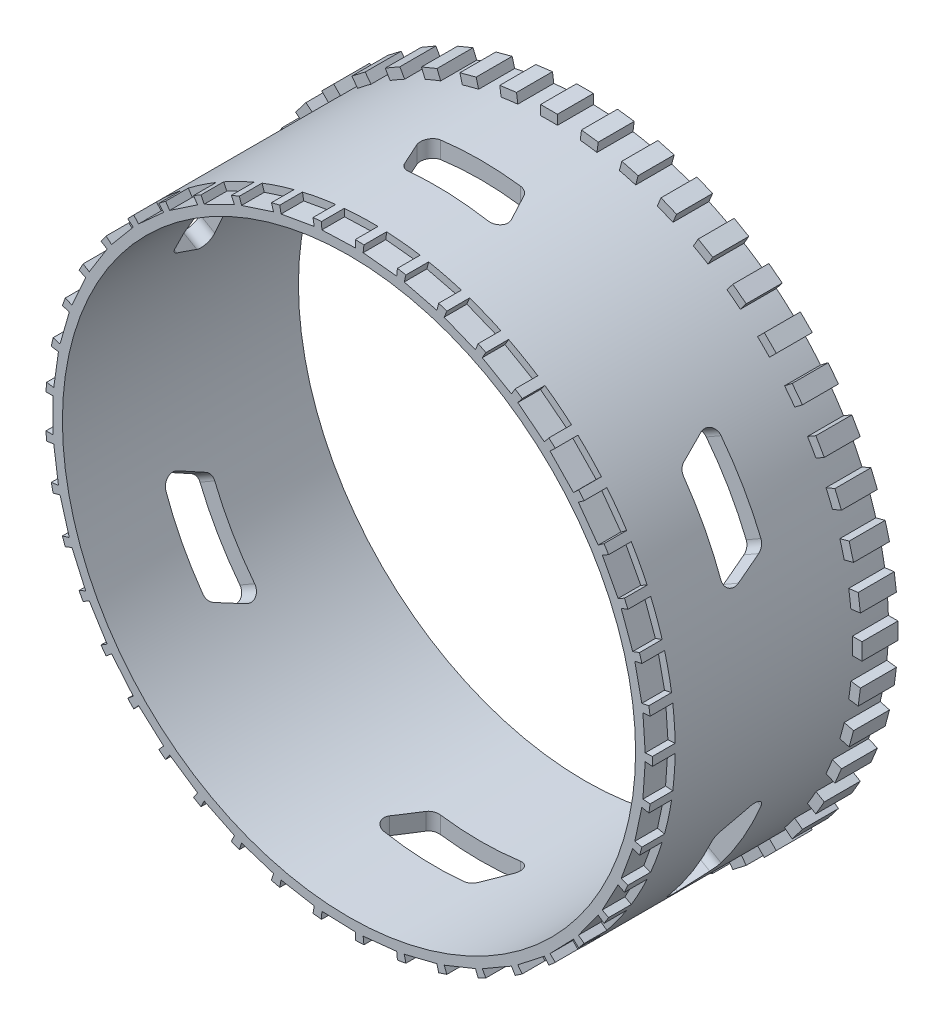
from build123d import *

# Parameters (mm, degrees)
SKETCH1_R           = 9
BOSS_EXTRUDE1_DEPTH = 7
SKETCH2_R           = 8.5
CUT_EXTRUDE1_DEPTH  = 10
CUT_EXTRUDE2_DEPTH  = 13
CIRPATTERN1_COUNT   = 6
SKETCH7_W           = 0.638695331
SKETCH7_H           = 1.067635278
BOSS_EXTRUDE2_DEPTH = 0.25
CIRPATTERN2_COUNT   = 48
SKETCH8_W           = 0.516008453
SKETCH8_H           = 1.064953617
CUT_EXTRUDE3_DEPTH  = 0.5
CIRPATTERN3_COUNT   = 45


with BuildPart() as part:
    # Sketch1 → Boss-Extrude1 (new body)
    with BuildSketch(Plane.XY):
        Circle(SKETCH1_R)
    extrude(amount=BOSS_EXTRUDE1_DEPTH)

    # Sketch2 → Cut-Extrude1 (cut)
    with BuildSketch(Plane.XY.offset(7)):
        Circle(SKETCH2_R)
    extrude(amount=-CUT_EXTRUDE1_DEPTH, mode=Mode.SUBTRACT)

    # Sketch6 → Cut-Extrude2 (cut)
    with BuildSketch(Plane(origin=(0, 0, 0), x_dir=(1, 0, 0), z_dir=(0, 1, 0))):
        with BuildLine():
            Line((1.183317486, -3.100815418), (-1.183317486, -3.100815418))
            ThreePointArc((-1.183317486, -3.100815418), (-1.341857532, -3.146129231), (-1.452503885, -3.268381727))
            Line((-1.452503885, -3.268381727), (-1.806713204, -3.988352079))
            ThreePointArc((-1.806713204, -3.988352079), (-1.792212991, -4.279325816), (-1.537526805, -4.42078577))
            Line((-1.537526805, -4.42078577), (0.829108167, -4.42078577))
            ThreePointArc((0.829108167, -4.42078577), (0.987648214, -4.375471956), (1.098294566, -4.253219461))
            Line((1.098294566, -4.253219461), (1.452503885, -3.533249109))
            ThreePointArc((1.452503885, -3.533249109), (1.438003672, -3.242275371), (1.183317486, -3.100815418))
        make_face()
    cut_extrude2 = extrude(amount=-CUT_EXTRUDE2_DEPTH, mode=Mode.SUBTRACT)

    # CirPattern1: Cut-Extrude2 ×6 about axis
    cirpattern1_axis = Axis((0, 0, 0), (0, 0, 1))
    for i in range(1, CIRPATTERN1_COUNT):
        add(cut_extrude2.rotate(cirpattern1_axis, i * 360 / CIRPATTERN1_COUNT), mode=Mode.SUBTRACT)

    # Sketch7 → Boss-Extrude2 (add, symmetric)
    with BuildSketch(Plane(origin=(0, 0, 0), x_dir=(1, 0, 0), z_dir=(0, 1, 0))):
        with Locations((-8.963024489, -0.533817639)):
            Rectangle(SKETCH7_W, SKETCH7_H)
    boss_extrude2 = extrude(amount=BOSS_EXTRUDE2_DEPTH, both=True)

    # CirPattern2: Boss-Extrude2 ×48 about axis
    cirpattern2_axis = Axis((0, 0, 0), (0, 0, 1))
    for i in range(1, CIRPATTERN2_COUNT):
        add(boss_extrude2.rotate(cirpattern2_axis, i * 360 / CIRPATTERN2_COUNT))

    # Sketch8 → Cut-Extrude3 (cut, symmetric)
    with BuildSketch(Plane(origin=(0, 0, 0), x_dir=(1, 0, 0), z_dir=(0, 1, 0))):
        with Locations((-9.030147935, -6.859544399)):
            Rectangle(SKETCH8_W, SKETCH8_H)
    cut_extrude3 = extrude(amount=CUT_EXTRUDE3_DEPTH, both=True, mode=Mode.SUBTRACT)

    # CirPattern3: Cut-Extrude3 ×45 about axis
    cirpattern3_axis = Axis((0, 0, 0), (0, 0, 1))
    for i in range(1, CIRPATTERN3_COUNT):
        add(cut_extrude3.rotate(cirpattern3_axis, i * 360 / CIRPATTERN3_COUNT), mode=Mode.SUBTRACT)


solid = part.part
